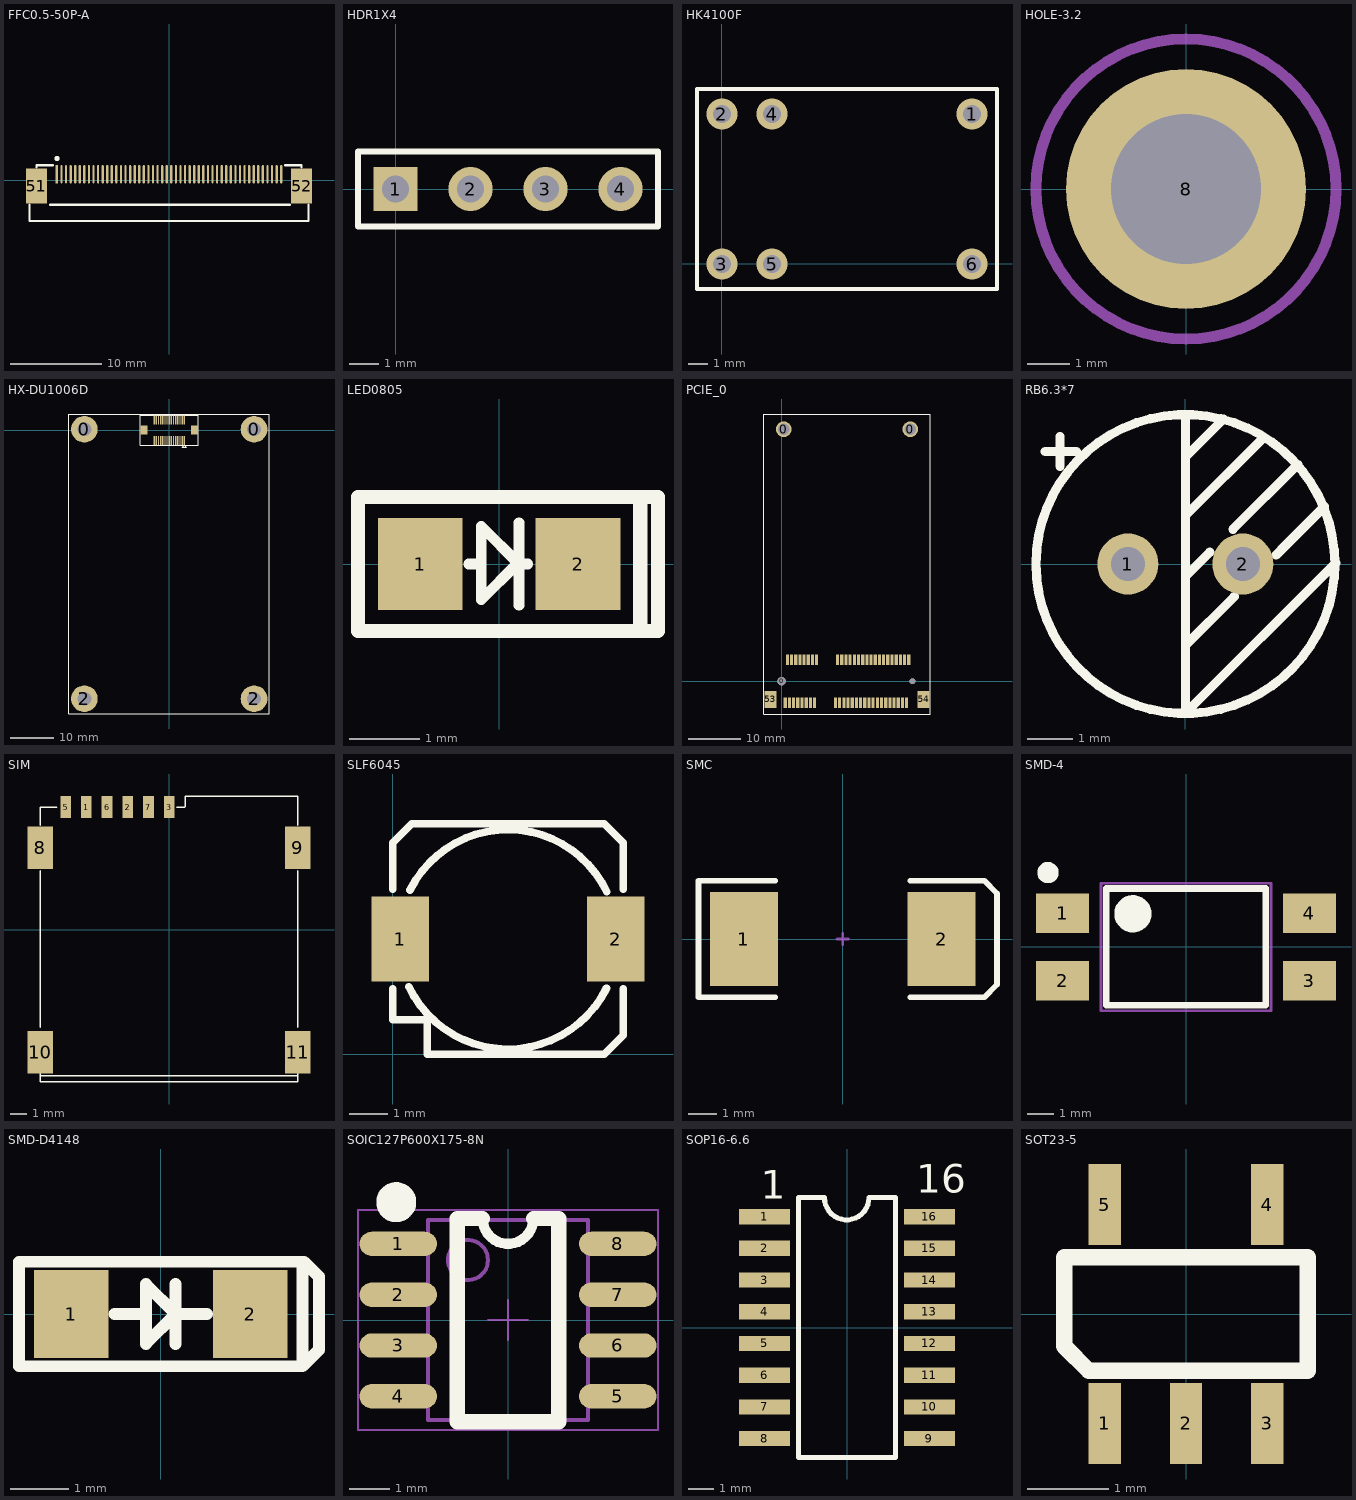
[diagram p0: the footprints below, top view; thin cyan lines are the x and y axes]
# Altium footprint library MISC84456-6.PcbLib: 41 footprints (part 2 of 3)
Each footprint in its own frame and in the unit in brackets; x right, y up, seen from the top. Pads: shape width x height; smd on the part's side, far side on the other; paste and mask are expansions set on the pad; w line width, h text height; cw(c..) or ccw(c..) is an arc to the next point about the centre after c.

## FFC0.5-50P-A [mm]
height 9.5
pads (52):
  rect 0.25x2 smd: 1(-12.246,0.645)
  oval 0.25x2 smd: 2(-11.746,0.645) 3(-11.246,0.645) 4(-10.746,0.645) 5(-10.246,0.645) 6(-9.746,0.645) 7(-9.246,0.645) 8(-8.746,0.645) 9(-8.246,0.645) 10(-7.746,0.645) 11(-7.246,0.645) 12(-6.746,0.645) 13(-6.246,0.645) 14(-5.746,0.645) 15(-5.246,0.645) 16(-4.746,0.645) 17(-4.246,0.645) 18(-3.746,0.645) 19(-3.246,0.645) 20(-2.746,0.645) 21(-2.246,0.645) 22(-1.746,0.645) 23(-1.246,0.645) 24(-0.746,0.645) 25(-0.246,0.645) 26(0.254,0.645) 27(0.754,0.645) 28(1.254,0.645) 29(1.754,0.645) 30(2.254,0.645) 31(2.754,0.645) 32(3.254,0.645) 33(3.754,0.645) 34(4.254,0.645) 35(4.754,0.645) 36(5.254,0.645) 37(5.754,0.645) 38(6.254,0.645) 39(6.754,0.645) 40(7.254,0.645) 41(7.754,0.645) 42(8.254,0.645) 43(8.754,0.645) 44(9.254,0.645) 45(9.754,0.645) 46(10.254,0.645) 47(10.754,0.645) 48(11.254,0.645) 49(11.754,0.645) 50(12.254,0.645)
  rect 2.286x3.81 smd: 51(-14.478,-0.645) 52(14.478,-0.645)
Top Overlay:
  circle w0.254: c-12.228,2.362 r0.163
  lines w0.254: -15.24,-2.677 -15.24,-4.455 15.24,-4.455 15.24,-2.677 ; -14.478,1.387 -14.478,1.641 -12.7,1.641 ; -12.954,-2.677 13.208,-2.677 ; 12.7,1.641 14.478,1.641 14.478,1.387

## HDR1X4 [mm] "Connector; Header; 4 Position"
pads (4):
  rect 1.5x1.5 hole 0.9: 1(0,0)
  round 1.5 hole 0.9: 2(2.54,0) 3(5.08,0) 4(7.62,0)
Top Overlay:
  lines w0.2: -1.27,-1.27 -1.27,1.27 8.89,1.27 8.89,-1.27 -1.27,-1.27

## HK4100F [mm] "11.8mm"
height 9.5
pads (6):
  round 1.6 hole 0.9: 1(12.7,7.62) 2(0,7.62) 3(0,0) 4(2.54,7.62) 5(2.54,0) 6(12.7,0)
Top Overlay:
  lines w0.2: -1.27,-1.27 13.97,-1.27 13.97,8.89 -1.27,8.89 -1.27,-1.27

## HOLE-3.2 [mm]
height 9.5
pads (1):
  round 5.6 hole 3.5: 8(0,0)
Mechanical 15:
  circle w0.254: c0,0 r3.5

## HX-DU1006D [mm]
pads (36):
  round 6.2 hole 3.2: 0(-19.75,0.23) 0(19.75,0.23) 2(-19.75,-62.51) 2(19.75,-62.51)
  rect 0.3x2.1 smd: 1(3.5,-2.35) 2(3.5,2.35) 3(3,-2.35) 4(3,2.35) 5(2.5,-2.35) 6(2.5,2.35) 7(2,-2.35) 8(2,2.35) 9(1.5,-2.35) 10(1.5,2.35) 11(1,-2.35) 12(1,2.35) 13(0.5,-2.35) 14(0.5,2.35) 15(0,-2.35) 16(0,2.35) 17(-0.5,-2.35) 18(-0.5,2.35) 19(-1,-2.35) 20(-1,2.35) 21(-1.5,-2.35) 22(-1.5,2.35) 23(-2,-2.35) 24(-2,2.35) 25(-2.5,-2.35) 26(-2.5,2.35) 27(-3,-2.35) 28(-3,2.35) 29(-3.5,-2.35) 30(-3.5,2.35)
  rect 1.6x2.1 smd: 31(-5.9,0) 31(5.9,0)
Top Overlay:
  lines w0.1: 3.476,-3.491 3.039,-3.928 3.928,-3.928 3.491,-3.491 ; -23.36,-66.07 -23.36,3.78 23.25,3.78 23.25,-66.07 -23.36,-66.07 ; -6.8,-3.5 6.8,-3.5 6.8,3.5 -6.8,3.5 -6.8,-3.5

## LED0805 [mm]
pads (2):
  rect 1.2x1.3 smd: 1(-1.118,0) 2(1.118,0)
Top Overlay:
  lines w0.152: -0.432,0 -0.254,0 ; 0.279,-0.584 0.279,0.584 ; 0.406,0 0.254,0 ; 0.254,0 -0.254,-0.508 -0.254,0.533 0.279,0 0.254,0
  lines w0.203: 1.93,-0.95 2.25,-0.95 2.25,0.95 2,0.95 ; 2,0.95 2,-0.95 -2,-0.95 -2,0.95 2,0.95

## PCIE_0 [mm]
height 3.98
pads (58):
  round 1.6 hole 1.6 unplated: 0(0,0)
  round 3 hole 2.2 unplated: 0(0.4,48.15) 0(24.6,48.15)
  round 1.1 hole 1.1 unplated: 0(25,0)
  rect 0.6x2 smd: 1(0.7,-4.1) 2(1.1,4.1) 3(1.5,-4.1) 4(1.9,4.1) 5(2.3,-4.1) 6(2.7,4.1) 7(3.1,-4.1) 8(3.5,4.1) 9(3.9,-4.1) 10(4.3,4.1) 11(4.7,-4.1) 12(5.1,4.1) 13(5.5,-4.1) 14(5.9,4.1) 15(6.3,-4.1) 16(6.7,4.1) 17(10.3,-4.1) 18(10.7,4.1) 19(11.1,-4.1) 20(11.5,4.1) 21(11.9,-4.1) 22(12.3,4.1) 23(12.7,-4.1) 24(13.1,4.1) 25(13.5,-4.1) 26(13.9,4.1) 27(14.3,-4.1) 28(14.7,4.1) 29(15.1,-4.1) 30(15.5,4.1) 31(15.9,-4.1) 32(16.3,4.1) 33(16.7,-4.1) 34(17.1,4.1) 35(17.5,-4.1) 36(17.9,4.1) 37(18.3,-4.1) 38(18.7,4.1) 39(19.1,-4.1) 40(19.5,4.1) 41(19.9,-4.1) 42(20.3,4.1) 43(20.7,-4.1) 44(21.1,4.1) 45(21.5,-4.1) 46(21.9,4.1) 47(22.3,-4.1) 48(22.7,4.1) 49(23.1,-4.1) 50(23.5,4.1) 51(23.9,-4.1) 52(24.3,4.1)
  rect 2.3x3.2 smd: 53(-2.15,-3.5) 54(27.15,-3.5)
Top Overlay:
  lines w0.1: -3.429,-6.275 -3.429,51.054 28.448,51.054 28.448,-6.275 -3.429,-6.275

## RB6.3*7 [mm]
pads (2):
  round 1.35 hole 0.75: 1(-1.27,0) 2(1.27,0)
Top Overlay:
  circle w0.203: c0,0 r3.302
  lines w0.203: -3.099,2.489 -2.413,2.489 ; -2.769,2.159 -2.769,2.819 ; 0,-1.8 1.079,-0.721 ; 0,-0.3 0,-0.28 0.539,0.259 ; 0,1.067 1.727,2.794 ; 0,2.362 0.838,3.2 ; 0,3.302 0,-3.302 3.327,0.025 ; 1.049,0.769 2.48,2.2 ; 2.003,0.2 3.073,1.27 2.134,0.33 2.13,0.33

## SIM [mm]
height 3.98
pads (10):
  rect 0.65x1.35 smd: 1(-5.07,7.512) 2(-2.53,7.512) 3(0.01,7.512) 5(-6.34,7.512) 6(-3.8,7.512) 7(-1.26,7.512)
  rect 1.55x2.6 smd: 8(-7.9,5.008) 9(7.9,5.008) 10(-7.9,-7.512) 11(7.9,-7.512)
Top Overlay:
  lines w0.1: -7.9,-8.962 7.9,-8.962 ; -7.9,-7.512 -7.9,-9.343 7.9,-9.343 7.9,-7.512 ; -7.9,-5.993 -7.9,3.611 ; -7.9,6.405 -7.9,7.512 -6.884,7.512 ; 0.482,7.512 0.955,7.512 0.99,7.548 0.99,8.183 7.9,8.183 7.9,6.405 ; 7.9,-5.993 7.9,3.611

## SLF6045 [mm]
height 3.98
pads (2):
  rect 1.5x2.2 smd: 1(0.2,3) 2(5.8,3)
Top Overlay:
  lines w0.2: 0,1.7 0,0.9 0.9,0.9 0.9,0 5.5,0 6,0.5 6,1.7 ; 0,4.3 0,5.5 0.5,6 5.5,6 6,5.5 6,4.3 ; 0.418,1.761 ccw(c3,3) 5.561,1.719 ; 0.454,4.273 cw(c3,3) 5.566,4.232

## SMC [mm] "DO-214-AB/SMC; 2 C-Bend Leads; Body 7.9 x 5.9 mm, inc. leads (LxW)"
height 2.65
pads (2):
  rect 2.4x3.3 smd: 1(-3.475,0) 2(3.475,0)
Top Overlay:
  lines w0.2: -2.375,-2.05 -5.075,-2.05 -5.075,2.05 -2.375,2.05 ; 2.375,-2.05 4.975,-2.05 5.425,-1.6 5.425,1.6 4.975,2.055 ; 2.375,2.05 4.975,2.05
Mechanical 1:
  lines w0.1: -0.2,0 0.2,0 ; 0,-0.2 0,0.2

## SMD-4 [mm]
height 9.5
pads (4):
  rect 2x1.5 smd: 1(-4.65,1.27) 2(-4.65,-1.27) 3(4.65,-1.27) 4(4.65,1.27)
Top Overlay:
  circle w0.4: c-5.2,2.8 r0.2
  circle w0.7: c-2,1.25 r0.35
  lines w0.254: -3,-2.2 -3,2.2 3,2.2 3,-2.2 -3,-2.2
Mechanical 13:
  lines w0.1: -3.2,-2.4 3.2,-2.4 3.2,2.4 -3.2,2.4 -3.2,-2.4
3D body: height 3.9, standoff 0, extent -5.015,-2.416 5.015,2.416

## SMD-D4148 [mm]
pads (2):
  rect 1.27x1.5 smd: 1(-1.524,0) 2(1.524,0)
Top Overlay:
  lines w0.203: -0.787,0 -0.254,0 ; 0.254,-0.508 0.254,0.508 ; 0.787,0 0.254,0 ; 0.254,0 -0.254,-0.508 -0.254,0.508 0.254,0 ; 2.413,-0.889 2.692,-0.61 2.692,0.635 2.438,0.889 2.413,0.889 ; 2.413,-0.889 2.413,0.889 ; 2.413,-0.889 -2.413,-0.889 -2.413,0.889 2.413,0.889

## SOIC127P600X175-8N [mil]
height 374.02
pads (8):
  oval 76.06x24 smd: 1(-108.03,75) 2(-108.03,25) 3(-108.03,-25) 4(-108.03,-75) 5(108.03,-75) 6(108.03,-25) 7(108.03,25) 8(108.03,75)
Top Overlay:
  circle w23.62: c-110,116 r7.87
  lines w10: -25,100 ccw(c0,100) 25,100
  lines w15: -25,100 -50,100 -50,-100 50,-100 50,100 25,100
Mechanical 15:
  circle w3.94: c-39.37,59.06 r19.68
  lines w3.94: -78.74,-98.43 78.74,-98.43 78.74,98.43 -78.74,98.43 -78.74,-98.43
  text "1" at 17.71,-6.47 h45
Mechanical 16:
  lines w0.04: -78.74,-98.43 78.74,-98.43 78.74,98.43 -78.74,98.43 -78.74,-98.43
  lines w1.97: -19.68,0 19.68,0 ; 0,-19.68 0,19.68 ; -147.64,-108.27 147.64,-108.27 147.64,108.27 -147.64,108.27 -147.64,-108.27
3D body: height 61.02, standoff -1.97, extent -117.91,-96 117.91,96.91

## SOP16-6.6 [mil]
height 374.02
pads (16):
  rect 80x24 smd: 1(-130,175) 2(-130,125) 3(-130,75) 4(-130,25) 5(-130,-25) 6(-130,-75) 7(-130,-125) 8(-130,-175) 9(130,-175) 10(130,-125) 11(130,-75) 12(130,-25) 13(130,25) 14(130,75) 15(130,125) 16(130,175)
Top Overlay:
  lines w8: -76.5,-205 -76.5,205 -35.59,205 ccw(c-0.5,205) 34.59,205 76.5,205 76.5,-205 -76.5,-205
  text "1" at -136,203 h45
  text "16" at 109,213 h45

## SOT23-5 [mm]
height 9.5
pads (5):
  rect 0.4x1 smd: 1(-1,-1.35) 2(0,-1.35) 3(1,-1.35) 4(1,1.35) 5(-1,1.35)
Top Overlay:
  lines w0.203: -1.5,-0.4 -1.2,-0.7 1.5,-0.7 1.5,-0.6 1.5,0.7 0,0.7 -1.5,0.7 -1.5,-0.3 -1.5,-0.4